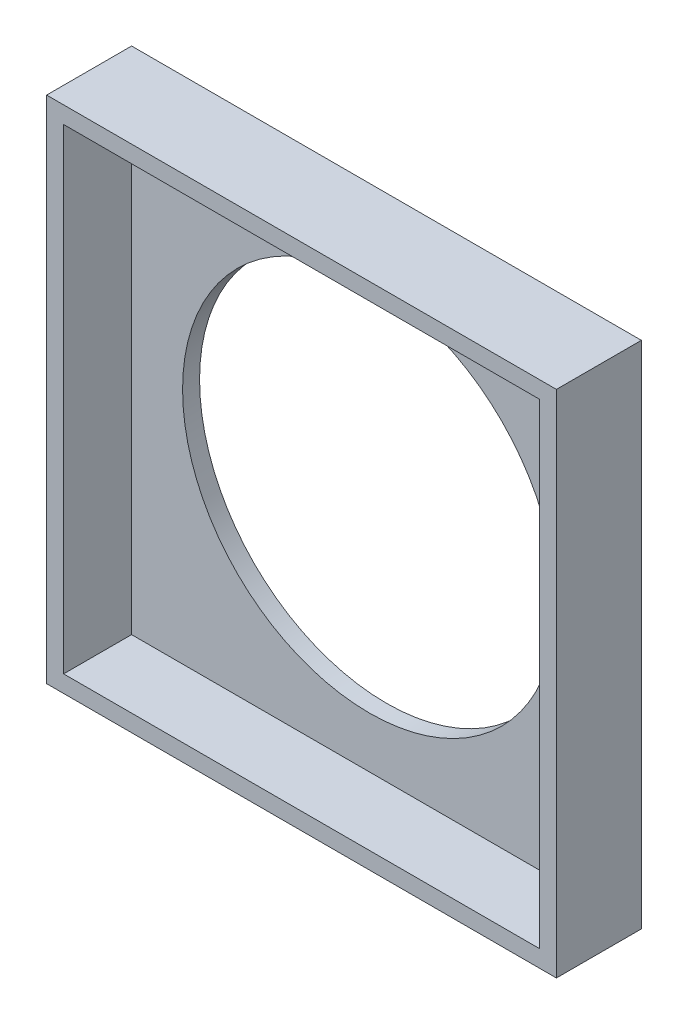
from build123d import *

# Parameters (mm, degrees)
SKETCH_1_3_W        = 28
SKETCH_1_3_H        = 28
BOSS_EXTRUDE1_DEPTH = 1
SKETCH_1_3_2_W      = 30
SKETCH_1_3_2_H      = 30
SKETCH_1_3_2_W_2    = 28
SKETCH_1_3_2_H_2    = 28
EXTRUDE_THIN1_DEPTH = 5
SKETCH2_R           = 11
CUT_EXTRUDE1_DEPTH  = 5


with BuildPart() as part:
    # Sketch 1_3 → Boss-Extrude1 (new body)
    with BuildSketch(Plane.XY):
        Rectangle(SKETCH_1_3_W, SKETCH_1_3_H)
    extrude(amount=BOSS_EXTRUDE1_DEPTH)

    # Sketch 1_3 2 → Extrude-Thin1 (add)
    with BuildSketch(Plane.XY):
        Rectangle(SKETCH_1_3_2_W, SKETCH_1_3_2_H)
        Rectangle(SKETCH_1_3_2_W_2, SKETCH_1_3_2_H_2, mode=Mode.SUBTRACT)
    extrude(amount=EXTRUDE_THIN1_DEPTH)

    # Sketch2 → Cut-Extrude1 (cut)
    with BuildSketch(Plane.XY.offset(1)):
        Circle(SKETCH2_R)
    extrude(amount=-CUT_EXTRUDE1_DEPTH, mode=Mode.SUBTRACT)


solid = part.part
